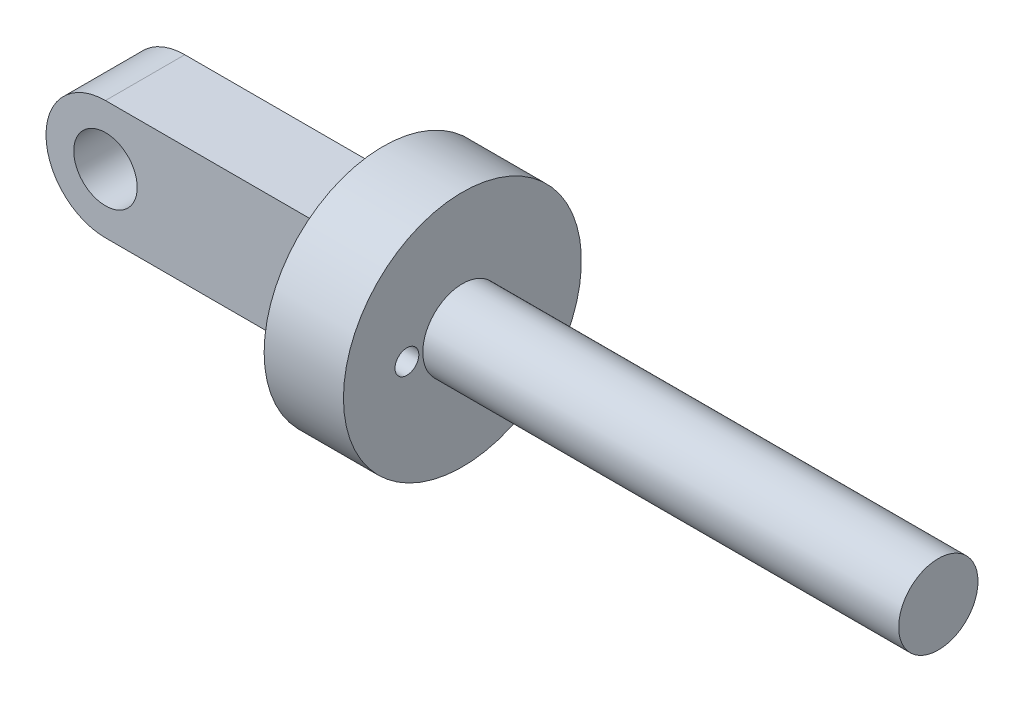
SolidWorks part; units mm, degrees
ref_plane "Front Plane" through (0, 0, 0) normal (0, 0, 1) x (1, 0, 0)
ref_plane "Top Plane" through (0, 0, 0) normal (0, 1, 0) x (1, 0, 0)
ref_plane "Right Plane" through (0, 0, 0) normal (1, 0, 0) x (0, 0, -1)
sketch "Sketch1" plane through (0, 0, 0) normal (0, 0, 1) x (1, 0, 0)
  line L0 (0, -60.0721) -> (0, 2943.5314) construction
  line L1 (0, 0) -> (0, 1.5)
  line L2 (0, 1.5) -> (1, 1.5)
  line L3 (1, 1.5) -> (1, 1)
  line L4 (1, 1) -> (7, 1)
  line L5 (7, 1) -> (7, 0)
  line L6 (0.1244, 0) -> (3003.7278, 0) construction
  line L7 (0, 0) -> (7, 0)
  point P8 (1, 1.25)
  dimension "D1" = 1
  dimension "D2" = 6
  dimension "D3" = 3
  dimension "D4" = 2
revolve "Revolve1" add sketch "Sketch1" angle 360 about L6
sketch "Sketch2" plane through (0, 0, 0) normal (0, 0, 1) x (1, 0, 0)
  line L0 (0, 0) -> (-50000, 0) construction
  line L1 (0, 0.75) -> (0, -0.75)
  line L2 (0, 1.5) -> (0, -1.5) construction
  line L3 (0, -0.75) -> (-3, -0.75)
  line L4 (0, 0) -> (0, 50000) construction
  line L5 (0, 0.75) -> (-3, 0.75)
  arc A0 (-3, -0.75) -> (-3, 0.75) centre (-3, 0) cw
  circle A1 centre (-3, 0) radius 0.4
  point P9 (0, 0)
  dimension "D1" = 0.75
  dimension "D3" = 0.8
  dimension "D2" = 3
extrude "Boss-Extrude1" add sketch "Sketch2" along normal mid plane 1
sketch "Sketch3" plane through (0, 0, 0) normal (0, 0, 1) x (1, 0, 0)
  line L0 (-1, 0.75) -> (-1, -0.75)
  line L1 (0, 0.75) -> (-3, 0.75) construction
  line L2 (-3, -0.75) -> (0, -0.75) construction
  line L3 (-1, -0.75) -> (-3, -0.75)
  line L4 (-3, 0.75) -> (-1, 0.75)
  line L5 (0, 1.5) -> (0, -1.5) construction
  arc A0 (-3, -0.75) -> (-3, 0.75) centre (-3, 0) cw
  dimension "D1" = 1
sketch "Sketch4" plane through (7, 0, 0) normal (1, 0, 0) x (0, 0, -1)
  circle A0 centre (0, 0) radius 0.5
  circle A1 centre (0, 0) radius 1
extrude "Cut-Extrude3" cut sketch "Sketch4" against normal blind 6
sketch "Sketch5" plane through (0, 0, 0) normal (-1, 0, 0) x (0, 0, 1)
  circle A0 centre (0.7, 0) radius 0.15
  dimension "D1" = 0.3
  dimension "D2" = 0.7
extrude "Cut-Extrude4" cut sketch "Sketch5" against normal blind 10
